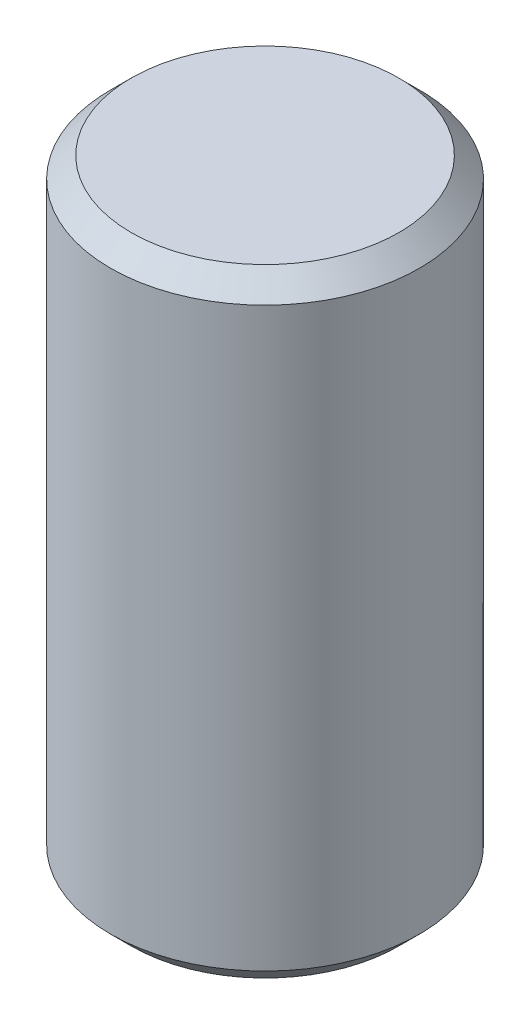
SolidWorks part; units mm, degrees
material "AISI 304"
ref_plane "Front Plane" through (0, 0, 0) normal (0, 0, 1) x (1, 0, 0)
ref_plane "Top Plane" through (0, 0, 0) normal (0, 1, 0) x (1, 0, 0)
ref_plane "Right Plane" through (0, 0, 0) normal (1, 0, 0) x (0, 0, -1)
sketch "Sketch1" plane through (0, 0, 0) normal (0, 1, 0) x (1, 0, 0)
  circle A0 centre (0, 0) radius 1.5
  dimension "D1" = 3
extrude "Boss-Extrude1" add sketch "Sketch1" along normal blind 6
chamfer "Chamfer1" distance 0.2 angle 45 2 edges at (0, 0, 1.5) (0, 6, 1.5)
